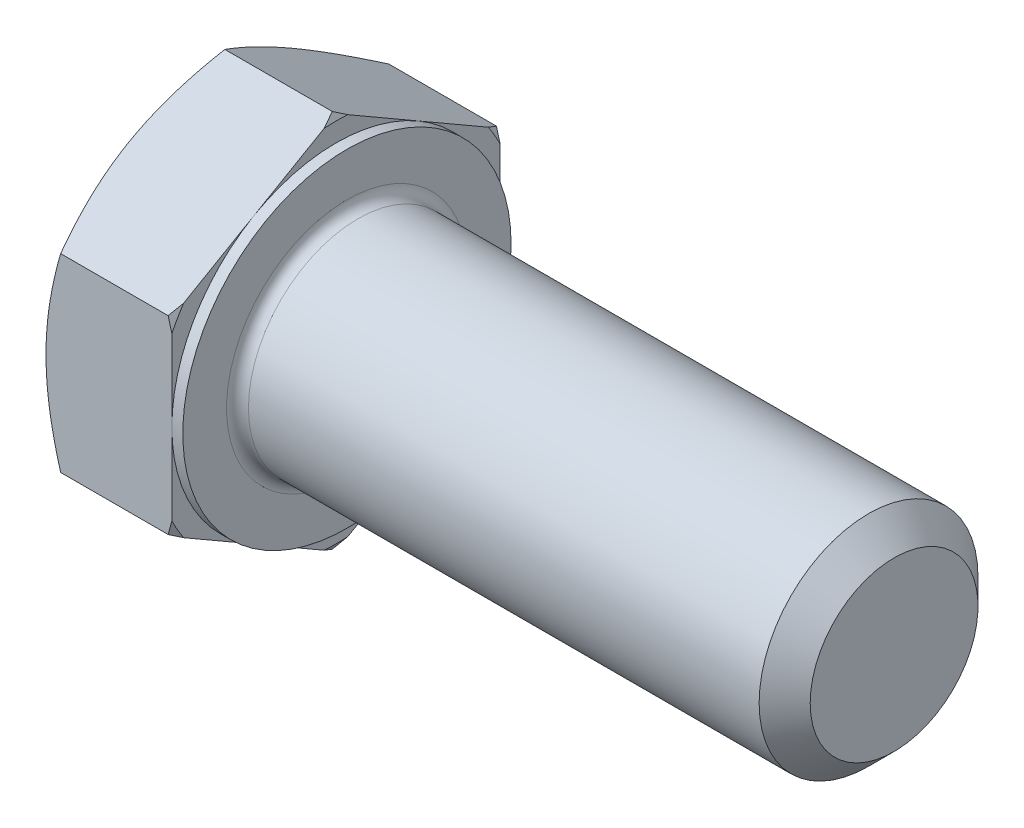
SolidWorks part; units mm, degrees
extrude "基体-拉伸" add sketch "草图1" along normal blind 7.5
sketch "草图1" plane through (0, 0, 0) normal (1, 0, 0) x (0, 0, -1)
  line L0 (9, 5.1962) -> (9, -5.1962)
  line L1 (-9, 5.1962) -> (-9, -5.1962)
  line L2 (9, -5.1962) -> (0, -10.3923)
  line L3 (0, -10.3923) -> (-9, -5.1962)
  line L4 (9, 5.1962) -> (0, 10.3923)
  line L5 (0, 10.3923) -> (-9, 5.1962)
revolve "切除-旋转1" cut sketch "草图3" angle 360 about L6
sketch "草图3" plane through (0, 0, 0) normal (0, 0, 1) x (1, 0, 0)
  line L0 (0, 9) -> (3.6906, 15.3923)
  line L1 (0, 10.3923) -> (0, 5.1962) construction
  line L2 (3.6906, 15.3923) -> (3.6906, 20.3923)
  line L3 (3.6906, 20.3923) -> (-10, 20.3923)
  line L4 (-10, 20.3923) -> (-10, 9)
  line L5 (-10, 9) -> (0, 9)
  line L6 (0, 0) -> (99.06, 0) construction
  line L7 (7.5, 10.3923) -> (0, 10.3923) construction
revolve "凸台-旋转1" add sketch "草图2" angle 360 about L7
sketch "草图2" plane through (0, 0, 0) normal (0, 0, 1) x (1, 0, 0)
  line L0 (0, 5.1962) -> (0, -5.1962) construction
  line L1 (0, 0) -> (37.5, 0)
  line L2 (0, 0) -> (0, 6)
  line L3 (0, 6) -> (37.5, 6)
  line L4 (37.5, 0) -> (37.5, 4.4845)
  line L5 (7.5, 10.3923) -> (7.5, 5.1962) construction
  line L7 (0, 0) -> (96.52, 0) construction
  line L8 (37.5, -4.4845) -> (90.335, -6) construction
  line L9 (0, -6) -> (90.335, -6) construction
  line L10 (9.25, 15.24) -> (9.25, -1.27) construction
  line L11 (7.5, 15.24) -> (7.5, -1.27) construction
  line L12 (7.5, 5.1962) -> (7.5, -5.1962) construction
  line L14 (37.5, 6) -> (37.5, 4.4845)
  dimension "l" = 30
  dimension "m" = 12
  dimension "Minor_dia" = 8.969
  dimension "p" = 1.75
  dimension "h" = 30
cosmetic thread "螺旋线1" parameters "Thread_length"=28.25, "Thread_minor"=8.969
material "3.6级"
ref_plane "前视" through (0, 0, 0) normal (0, 0, 1) x (1, 0, 0)
ref_plane "上视" through (0, 0, 0) normal (0, 1, 0) x (1, 0, 0)
ref_plane "右视" through (0, 0, 0) normal (1, 0, 0) x (0, 0, -1)
sketch "草图5" plane through (0, 0, 0) normal (0, 0, 1) x (1, 0, 0)
  line L0 (7.5, 9) -> (3.8094, 15.3923)
  line L1 (7.5, 10.3923) -> (7.5, 5.1962) construction
  line L2 (3.8094, 15.3923) -> (3.8094, 20.3923)
  line L3 (3.8094, 20.3923) -> (13.8094, 20.3923)
  line L4 (13.8094, 20.3923) -> (13.8094, 9)
  line L5 (13.8094, 9) -> (7.5, 9)
  line L7 (7.5, 10.3923) -> (0.8038, 10.3923) construction
  line L8 (0, 0) -> (99.06, 0) construction
  line L9 (0, 0) -> (99.06, 0) construction
revolve "切除-旋转2" cut sketch "草图5" angle 360 about L8
sketch "草图4" plane through (0, 0, 0) normal (0, 0, 1) x (1, 0, 0)
  line L1 (7.5, 10.3923) -> (7.5, 5.1962) construction
  line L2 (7.5, 9) -> (6.9, 9)
  line L3 (7.5, 9) -> (7.5, 20.3923)
  line L4 (7.5, 20.3923) -> (6.9, 20.3923)
  line L5 (0, 0) -> (95.25, 0) construction
  line L6 (0, 0) -> (96.52, 0) construction
  line L7 (6.9, 9) -> (6.9, 20.3923)
  line L8 (6.6962, 10.3923) -> (0.8038, 10.3923) construction
revolve "切除-旋转3" cut sketch "草图4" angle 360 about L5
chamfer "倒角" distance 1.4 angle 45 1 edges at (37.5, 0, 6)
fillet "圆角" radius 0.6 1 edges at (7.5, 0, -6)
sketch "草图6" plane through (0, 0, 0) normal (0, 0, 1) x (1, 0, 0)
  line L0 (8.975, -4.4845) -> (8.1, -6)
  line L1 (8.975, -4.4845) -> (9.8499, -6)
  line L2 (9.8499, -6) -> (9.8499, -7.5)
  line L3 (-3.175, 0) -> (5.1513, 0) construction
  line L5 (9.8499, -7.5) -> (8.1, -7.5)
  line L6 (8.1, -7.5) -> (8.1, -6)
  arc A0 (8.1, -6) -> (7.5, -6.6) centre (8.1, -6.6) ccw construction
revolve "切除-旋转4" [suppressed] cut sketch "草图6" angle 360 about L3
pattern_linear "阵列(线性)1" [suppressed]
equation "\"D3@草图1\" = \"s@草图1\" / 2"
equation "\"D4@草图1\" = \"D3@草图1\""
equation "\"D5@草图1\" = \"D4@草图1\""
equation "\"D1@草图3\" = \"s@草图1\" / 2"
equation "\"D1@草图5\" = \"s@草图1\" / 2"
equation "\"Head_ch_ang@草图5\" = \"Head_ch_ang@草图3\""
equation "\"D1@草图4\" = \"s@草图1\""
equation "\"Diameter@草图6\" = \"m@草图2\""
equation "\"Overcut@草图6\" = \"m@草图2\" * 1.25"
equation "\"Minor_dia@草图2\" = \"m@草图2\"-\"p@草图2\" * 1.732"
equation "\"Thread_minor@螺旋线1\" = \"Minor_dia@草图2\""
equation "\"Thread_minor@草图6\" = \"Minor_dia@草图2\""
equation "\"D1@倒角\" = \"p@草图2\"*0.8"
equation "\"Thread_length@螺旋线1\" = \"l@草图2\" - \"p@草图2\""
equation "\"Num_threads@阵列(线性)1\" = \"l@草图2\" / \"p@草图2\""
